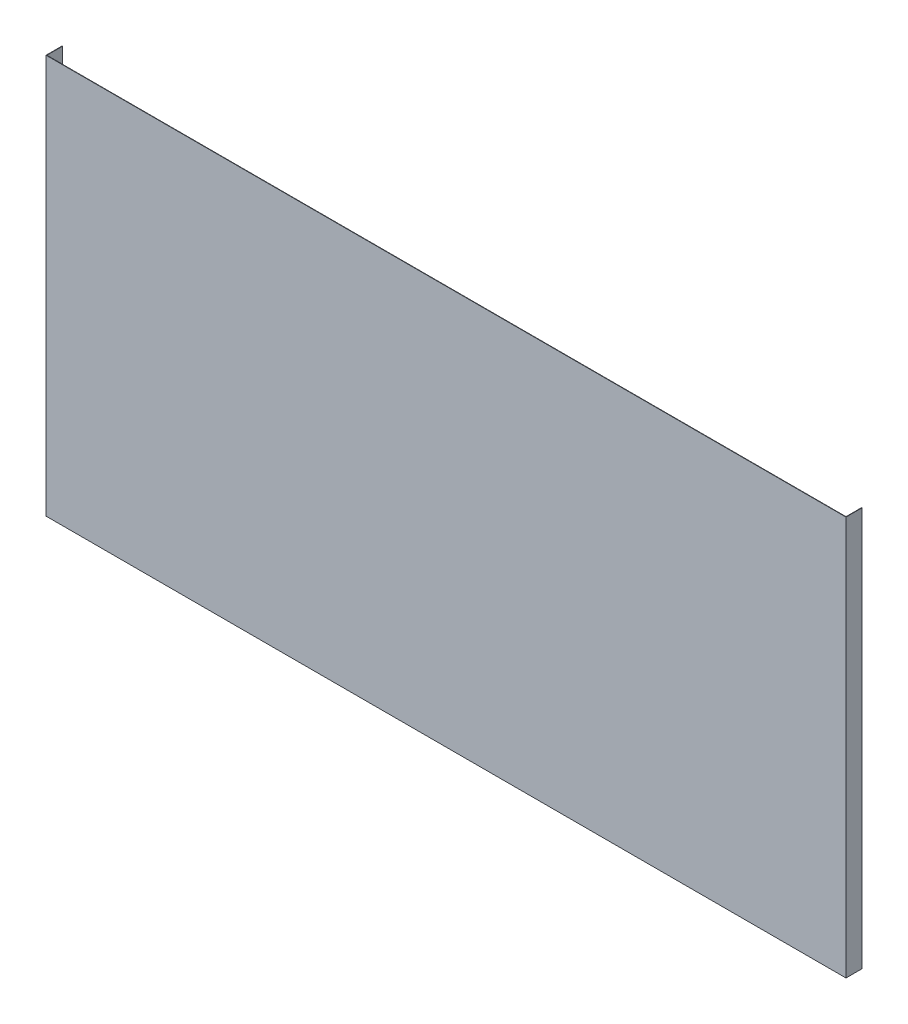
from build123d import *

# Parameters (mm, degrees)
SKETCH_1_W      = 4004
SKETCH_1_H      = 2000
EXTRUDE_1_DEPTH = 2
SKETCH_2_W      = 80
SKETCH_2_H      = 2000
EXTRUDE_2_DEPTH = 2
SKETCH_3_W      = 80
SKETCH_3_H      = 2000
EXTRUDE_3_DEPTH = 2


with BuildPart() as part:
    # 草图1 → 凸台-拉伸1 (new body)
    with BuildSketch(Plane.XY):
        Rectangle(SKETCH_1_W, SKETCH_1_H)
    extrude(amount=EXTRUDE_1_DEPTH)

    # 草图2 → 凸台-拉伸2 (add)
    with BuildSketch(Plane.ZY.offset(2002)):
        with Locations((-38, 0)):
            Rectangle(SKETCH_2_W, SKETCH_2_H)
    extrude(amount=EXTRUDE_2_DEPTH)

    # 草图3 → 凸台-拉伸3 (add)
    with BuildSketch(Plane(origin=(2002, 0, 0), x_dir=(0, 0, -1), z_dir=(1, 0, 0))):
        with Locations((38, 0)):
            Rectangle(SKETCH_3_W, SKETCH_3_H)
    extrude(amount=EXTRUDE_3_DEPTH)


solid = part.part
